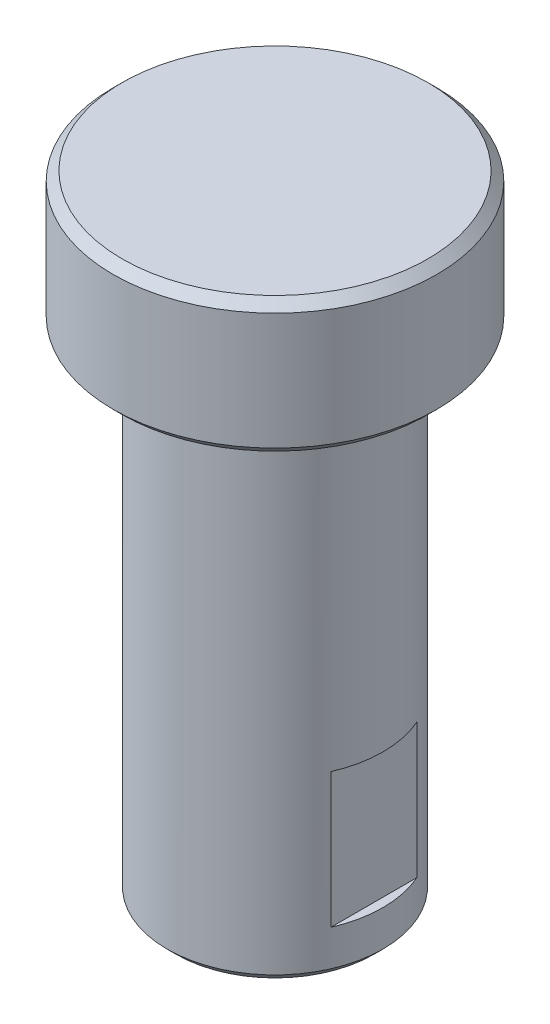
SolidWorks part; units mm, degrees
ref_plane "Front Plane" through (0, 0, 0) normal (0, 0, 1) x (1, 0, 0)
ref_plane "Top Plane" through (0, 0, 0) normal (0, 1, 0) x (1, 0, 0)
ref_plane "Right Plane" through (0, 0, 0) normal (1, 0, 0) x (0, 0, -1)
sketch "Sketch2" plane through (0, 0, 0) normal (0, 0, 1) x (1, 0, 0)
  line L0 (0, 14.1064) -> (0, -21.3459) construction
  line L1 (0, 48.6541) -> (-18, 48.6541)
  line L2 (-18, 48.6541) -> (-18, 33.6541)
  line L3 (-18, 33.6541) -> (-12, 33.6541)
  line L4 (-12, 33.6541) -> (-12, -21.3459)
  line L5 (-12, -21.3459) -> (0, -21.3459)
  line L6 (0, -21.3459) -> (0, 48.6541)
  dimension "D1" = 18
  dimension "D2" = 12
  dimension "D3" = 15
  dimension "D4" = 70
revolve "Revolve1" add sketch "Sketch2" angle 360 about L0
chamfer "Chamfer1" distance 1 angle 45 3 edges at (0, -21.3459, 12) (0, 33.6541, 18) (0, 48.6541, 18)
sketch "Sketch3" plane through (0, 0, 0) normal (0, 0, 1) x (1, 0, 0)
  line L0 (-12, 33.6541) -> (-12, -20.3459) construction
  line L1 (-12, -1.3459) -> (-11, -1.3459)
  line L2 (-12, -1.3459) -> (-12, -16.3459)
  line L3 (-12, -16.3459) -> (-11, -16.3459)
  line L4 (-11, -1.3459) -> (-11, -16.3459)
  line L5 (17, 48.6541) -> (-17, 48.6541) construction
  line L7 (0, 0) -> (0, -26.3881) construction
  line L8 (11, -1.3459) -> (11, -16.3459)
  line L9 (12, -16.3459) -> (11, -16.3459)
  line L10 (12, -1.3459) -> (12, -16.3459)
  line L11 (12, -1.3459) -> (11, -1.3459)
  dimension "D1" = 50
  dimension "D2" = 15
  dimension "D3" = 1
extrude "Cut-Extrude1" cut sketch "Sketch3" against normal through all both and the other way through all
hole_wizard "M14x1.5 Tapped Hole1" positions "Sketch4" profile "Sketch5" tap size "M14x1.5" standard "GB"
sketch "Sketch4" plane through (0, -21.3459, 0) normal (0, -1, 0) x (-1, 0, 0)
  point P0 (0, 0)
sketch "Sketch5" plane through (0, -21.3459, 0) normal (1, 0, 0) x (0, 0, -1)
  line L0 (0, 0) -> (0, 23.7554)
  line L1 (0, 23.7554) -> (6.25, 20)
  line L2 (6.25, 20) -> (6.25, 0)
  line L5 (6.25, 0) -> (0, 0)
  line L10 (0, 23.7554) -> (-6.25, 20) construction
  line L11 (0, -6.35) -> (0, 107.95) construction
  dimension "螺纹孔钻头直径" = 12.5
  dimension "螺纹孔钻头深度" = 20
  dimension "导头角度" = 118
cosmetic thread "Cosmetic thread 1" parameters "D1"=20, "D2"=14
